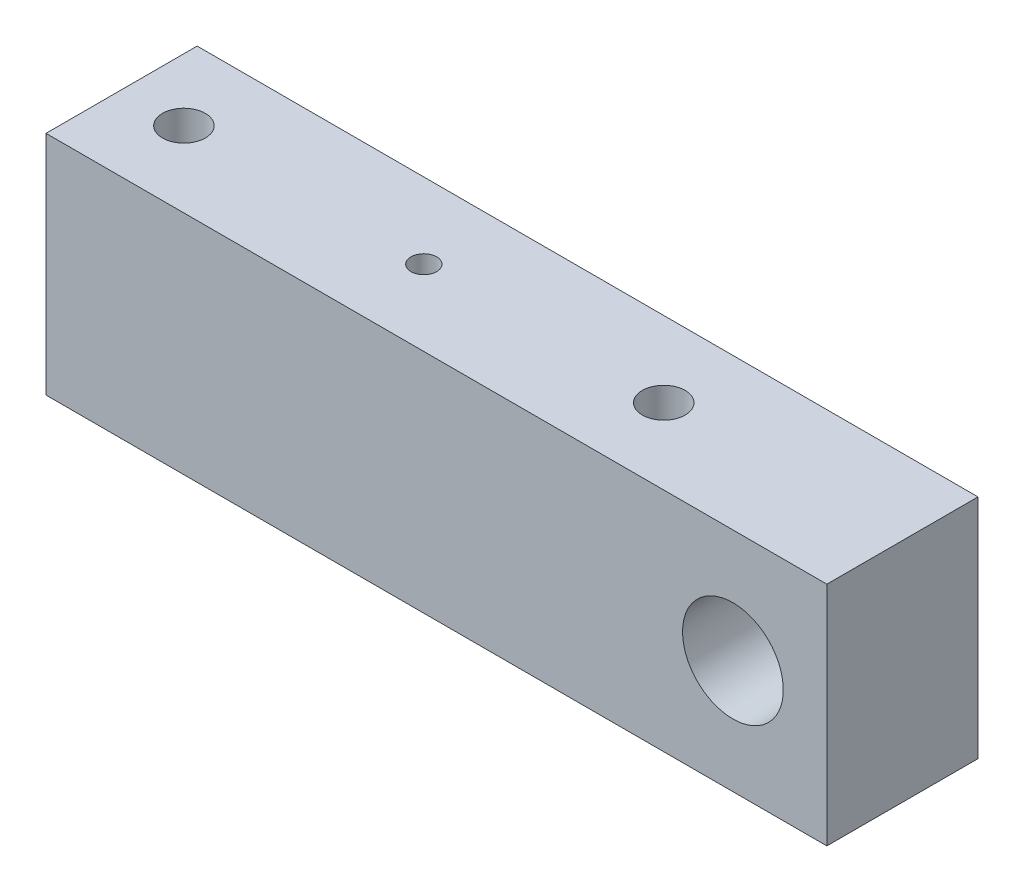
SolidWorks part; units mm, degrees
material "1023 碳钢板 (SS)"
ref_plane "前视基准面" through (0, 0, 0) normal (0, 0, 1) x (1, 0, 0)
ref_plane "上视基准面" through (0, 0, 0) normal (0, 1, 0) x (1, 0, 0)
ref_plane "右视基准面" through (0, 0, 0) normal (1, 0, 0) x (0, 0, -1)
sketch "草图1" plane through (0, 0, 0) normal (0, 0, 1) x (1, 0, 0)
  line L1 (155, 45) -> (-155, 45)
  line L2 (155, 45) -> (155, -45)
  line L3 (155, -45) -> (-155, -45)
  line L4 (-155, 45) -> (-155, -45)
  line L5 (155, 45) -> (-155, -45) construction
  line L6 (155, -45) -> (-155, 45) construction
  point P0 (0, 0)
  dimension "D1" = 310
  dimension "D2" = 90
extrude "凸台-拉伸1" add sketch "草图1" along normal blind 60
sketch "草图2" plane through (0, 45, 0) normal (0, 1, 0) x (1, 0, 0)
  line L0 (155, 0) -> (-155, 0) construction
  line L1 (-155, -60) -> (-155, 0) construction
  circle A0 centre (-130.25, -30) radius 8.5
  circle A1 centre (60.25, -30) radius 8.5
  point P6 (0, 0)
  dimension "D2" = 17
  dimension "D4" = 24.75
  dimension "D1" = 190.5
  dimension "D3" = 30
extrude "切除-拉伸1" cut sketch "草图2" against normal blind 90
sketch "草图3" plane through (0, 45, 0) normal (0, 1, 0) x (1, 0, 0)
  line L0 (155, 0) -> (-155, 0) construction
  circle A0 centre (-35, -30) radius 7.9239
  circle A1 centre (-130.25, -30) radius 8.5 construction
  point P6 (0, 0)
  dimension "D2" = 30
  dimension "D1" = 95.25
hole_wizard "M12 螺纹孔1" positions "草图4" profile "草图5" tap size "M12" standard "ISO"
sketch "草图4" plane through (0, 45, 0) normal (0, 1, 0) x (1, 0, 0)
  point P0 (-35, -30)
sketch "草图5" plane through (-35, 45, 30) normal (1, 0, 0) x (0, 0, 1)
  line L0 (0, 0) -> (0, 33.3144)
  line L1 (0, 33.3144) -> (5.1, 30.25)
  line L2 (5.1, 30.25) -> (5.1, 0)
  line L5 (5.1, 0) -> (0, 0)
  line L10 (0, 33.3144) -> (-5.1, 30.25) construction
  line L11 (0, -6.35) -> (0, 107.95) construction
  dimension "螺纹孔钻头直径" = 10.2
  dimension "螺纹孔钻头深度" = 30.25
  dimension "导头角度" = 118
cosmetic thread "孔螺蚊线1" parameters "D1"=25, "D2"=12
sketch "草图6" plane through (0, 0, 0) normal (0, 0, -1) x (-1, 0, 0)
  line L0 (-155, -45) -> (-155, 45) construction
  circle A0 centre (-117.7, 0) radius 20
  dimension "D1" = 40
  dimension "D2" = 37.3
extrude "切除-拉伸2" cut sketch "草图6" against normal blind 60
